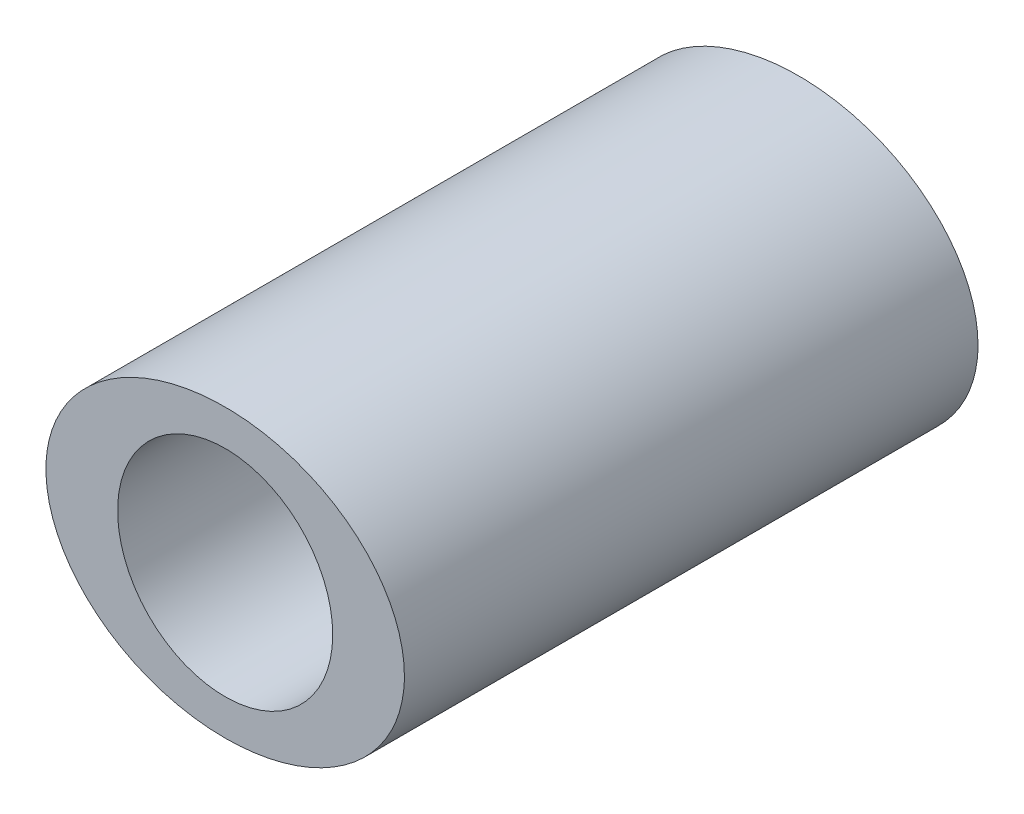
SolidWorks part; units mm, degrees
material "Q235A"
ref_plane "Front Plane" through (0, 0, 0) normal (0, 0, 1) x (1, 0, 0)
ref_plane "Top Plane" through (0, 0, 0) normal (0, 1, 0) x (1, 0, 0)
ref_plane "Right Plane" through (0, 0, 0) normal (1, 0, 0) x (0, 0, -1)
sketch "Sketch1" plane through (0, 0, 0) normal (0, 0, 1) x (1, 0, 0)
  ellipse E0 centre (0, 0) end of major axis (25, 0) minor radius 20
  dimension "D1" = 25
  dimension "D2" = 20
extrude "Boss-Extrude1" add sketch "Sketch1" along normal mid plane 80
sketch "Sketch2" plane through (0, 0, 40) normal (0, 0, 1) x (1, 0, 0)
  circle A0 centre (0, 0) radius 15
  dimension "D1" = 30
extrude "Cut-Extrude1" cut sketch "Sketch2" against normal through all
sketch "Sketch3" plane through (0, 0, 40) normal (0, 0, 1) x (1, 0, 0)
  line L0 (-25, 0) -> (25, 0)
  ellipse E0 centre (0, 0) end of major axis (25, 0) minor radius 20 construction
